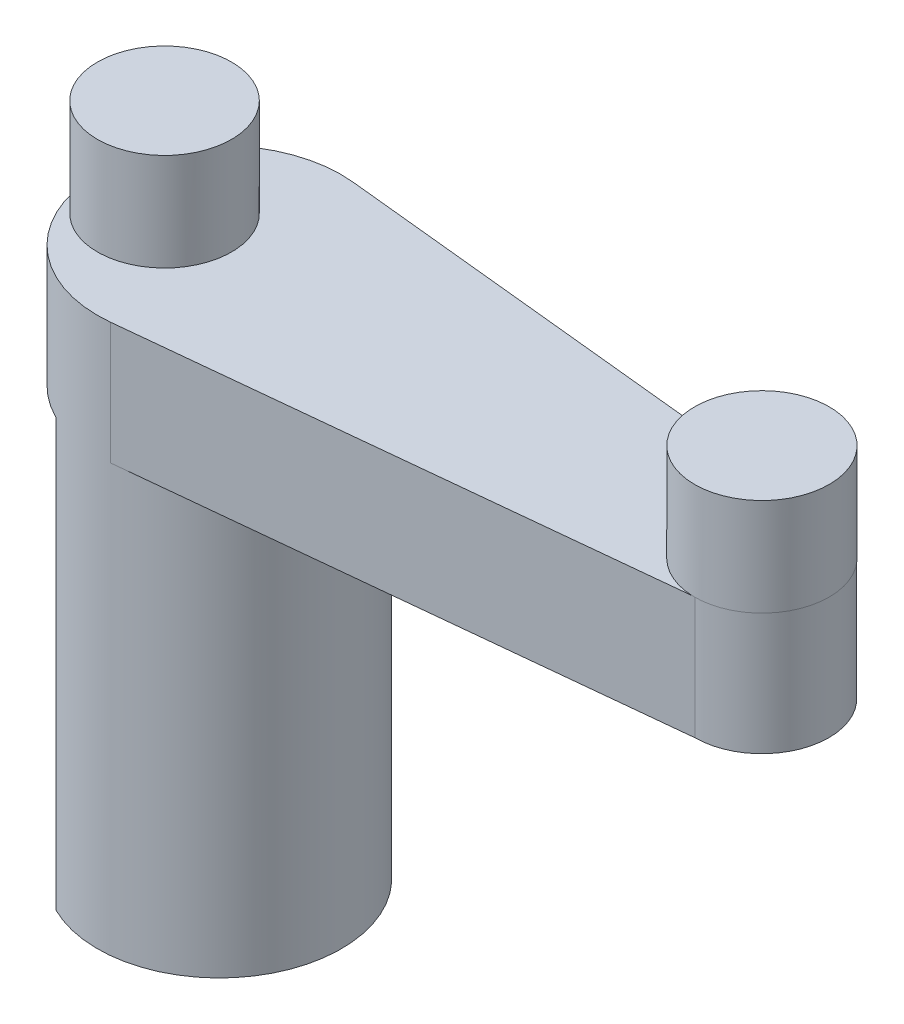
SolidWorks part; units mm, degrees
ref_plane "前视基准面" through (0, 0, 0) normal (0, 0, 1) x (1, 0, 0)
ref_plane "上视基准面" through (0, 0, 0) normal (0, 1, 0) x (1, 0, 0)
ref_plane "右视基准面" through (0, 0, 0) normal (1, 0, 0) x (0, 0, -1)
sketch "草图1" plane through (0, 0, 0) normal (0, 1, 0) x (1, 0, 0)
  line L0 (-1, 2.7091) -> (-1, -1.7636) construction
  line L1 (5, -1) -> (5, 0.55) construction
  line L2 (0.1018, -0.9948) -> (4.45, -0.55)
  line L3 (0.1018, 0.9948) -> (4.45, 0.55)
  arc A0 (0.1018, 0.9948) -> (0.1018, -0.9948) centre (0, 0) ccw
  arc A1 (4.45, -0.55) -> (4.45, 0.55) centre (4.45, 0) ccw
  dimension "D1" = 2
  dimension "D2" = 1.1
  dimension "D3" = 6
extrude "凸台-拉伸1" add sketch "草图1" along normal blind 1
sketch "草图2" plane through (0, 1, 0) normal (0, 1, 0) x (1, 0, 0)
  circle A0 centre (4.45, 0) radius 0.5521
  circle A1 centre (-0.45, 0) radius 0.55
  arc A2 (0.1018, 0.9948) -> (0.1018, -0.9948) centre (0, 0) ccw construction
  dimension "D1" = 1.1
extrude "凸台-拉伸2" add sketch "草图2" along normal blind 0.8
sketch "草图3" plane through (0, 0, 0) normal (0, -1, 0) x (1, 0, 0)
  line L0 (0.2588, -0.9659) -> (-0.1812, 0.6761)
  line L1 (0, -1.2974) -> (0, 1.332) construction
  line L3 (-0.3744, 0.6244) -> (-0.1812, 0.6761)
  line L4 (-0.3744, 0.6244) -> (-0.4468, 0.8946)
  arc A0 (0.2588, -0.9659) -> (-0.4468, 0.8946) centre (0, 0) ccw
  point P7 (0.0656, -1.0177)
  point P8 (-0.452, 0.9142)
  dimension "D1" = 15
extrude "凸台-拉伸3" add sketch "草图3" along normal blind 3.5
scale "缩放比例1" scale about centroid uniform scaling yes scale factor 0.7
